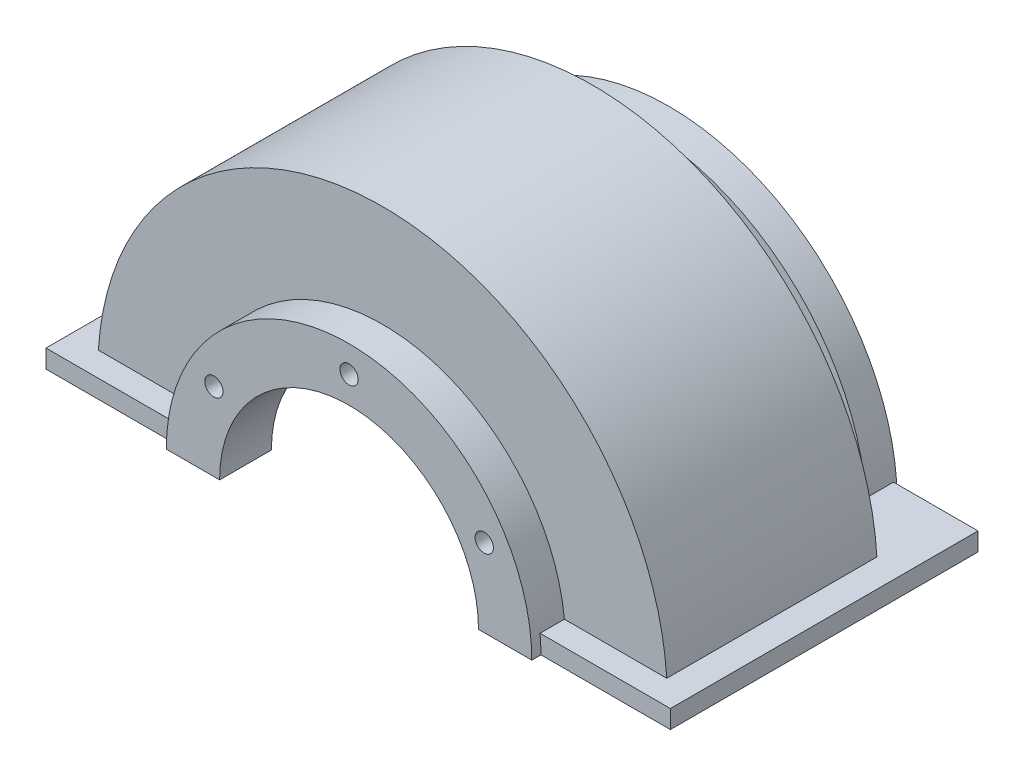
from build123d import *

# Parameters (mm, degrees)
BOSS_EXTRUDE1_DEPTH            = 202
CUT_EXTRUDE1_START             = -16
CUT_EXTRUDE1_DEPTH             = 16
CUT_EXTRUDE2_DEPTH             = 18
CUT_EXTRUDE3_DEPTH             = 30
BOSS_EXTRUDE2_START            = 2
BOSS_EXTRUDE2_DEPTH            = 2
BOSS_EXTRUDE3_DEPTH            = 6
BOSS_EXTRUDE4_DEPTH            = 30
F_16_0_16_DIAMETER_HOLE1_D     = 16
F_16_0_16_DIAMETER_HOLE1_DEPTH = 20
F_12_0_12_DIAMETER_HOLE1_D     = 12
F_12_0_12_DIAMETER_HOLE1_DEPTH = 34


with BuildPart() as part:
    # Sketch1 → Boss-Extrude1 (new body)
    with BuildSketch(Plane(origin=(0, 0, -358.692981355), x_dir=(-1, 0, 0), z_dir=(0, 0, -1))):
        with BuildLine():
            Line((-707.84521865, 246.743963655), (-726.230642584, 246.743963655))
            Line((-726.230642584, 246.743963655), (-726.230642584, 234.743963655))
            Line((-726.230642584, 234.743963655), (-316.230642584, 234.743963655))
            Line((-316.230642584, 234.743963655), (-316.230642584, 246.743963655))
            Line((-316.230642584, 246.743963655), (-334.616066519, 246.743963655))
            ThreePointArc((-334.616066519, 246.743963655), (-521.230642584, 421.743963655), (-707.84521865, 246.743963655))
        make_face()
    extrude(amount=-BOSS_EXTRUDE1_DEPTH)

    # Sketch2 → Cut-Extrude1 (cut)
    with BuildSketch(Plane.XY.offset(-156.692981355).offset(CUT_EXTRUDE1_START)):
        with BuildLine():
            Line((640.629135037, 246.743963655), (707.84521865, 246.743963655))
            ThreePointArc((707.84521865, 246.743963655), (521.230642584, 421.743963655), (334.616066519, 246.743963655))
            Line((334.616066519, 246.743963655), (401.832150132, 246.743963655))
            ThreePointArc((401.832150132, 246.743963655), (521.230642584, 354.743963655), (640.629135037, 246.743963655))
        make_face()
    extrude(amount=CUT_EXTRUDE1_DEPTH, mode=Mode.SUBTRACT)

    # Sketch3 → Cut-Extrude2 (cut)
    with BuildSketch(Plane(origin=(0, 0, -358.692981355), x_dir=(-1, 0, 0), z_dir=(0, 0, -1))):
        with BuildLine():
            Line((-371.711413052, 246.743963655), (-334.616066519, 246.743963655))
            ThreePointArc((-334.616066519, 246.743963655), (-521.230642584, 421.743963654), (-707.84521865, 246.743963655))
            Line((-707.84521865, 246.743963655), (-670.749872117, 246.743963655))
            ThreePointArc((-670.749872117, 246.743963655), (-521.230642584, 384.743963654), (-371.711413052, 246.743963655))
        make_face()
    extrude(amount=-CUT_EXTRUDE2_DEPTH, mode=Mode.SUBTRACT)

    # Sketch4 → Cut-Extrude3 (cut)
    with BuildSketch(Plane(origin=(0, 0, -340.692981355), x_dir=(-1, 0, 0), z_dir=(0, 0, -1))):
        with BuildLine():
            Line((-707.84521865, 246.743963655), (-334.616066519, 246.743963655))
            ThreePointArc((-334.616066519, 246.743963655), (-521.230642584, 421.743963655), (-707.84521865, 246.743963655))
        make_face()
    extrude(amount=-CUT_EXTRUDE3_DEPTH, mode=Mode.SUBTRACT)

    # Sketch5 → Boss-Extrude2 (add)
    with BuildSketch(Plane(origin=(0, 0, -358.692981355), x_dir=(-1, 0, 0), z_dir=(0, 0, -1)).offset(BOSS_EXTRUDE2_START)):
        with BuildLine():
            Line((-371.230642584, 234.743963655), (-671.230642584, 234.743963655))
            ThreePointArc((-671.230642584, 234.743963655), (-521.230642584, 384.743963655), (-371.230642584, 234.743963655))
        make_face()
    extrude(amount=-BOSS_EXTRUDE2_DEPTH)

    # Sketch6 → Boss-Extrude3 (add)
    with BuildSketch(Plane.XY.offset(-156.692981355)):
        with BuildLine():
            Line((641.230642584, 234.743963655), (401.230642584, 234.743963655))
            ThreePointArc((401.230642584, 234.743963655), (521.230642584, 354.743963655), (641.230642584, 234.743963655))
        make_face()
    extrude(amount=BOSS_EXTRUDE3_DEPTH)

    # Sketch7 → Boss-Extrude4 (add)
    with BuildSketch(Plane.XY.offset(-340.692981355)):
        with BuildLine():
            Line((619.500678709, 246.743963655), (422.960606459, 246.743963655))
            ThreePointArc((422.960606459, 246.743963655), (521.230642584, 333.743963655), (619.500678709, 246.743963655))
        make_face()
    extrude(amount=BOSS_EXTRUDE4_DEPTH)

    # Sketch8 → Cut-Revolve1 (revolve, cut)
    with BuildSketch(Plane(origin=(0, 234.743963655, 0), x_dir=(1, 0, 0), z_dir=(0, 1, 0))):
        Polygon((606.230642584, 360.692981355), (521.230642584, 360.692981355), (521.230642584, 150.692981355), (606.230642584, 150.692981355), (606.230642584, 184.692981355), (696.230642584, 184.692981355), (696.230642584, 298.692981355), (606.230642584, 298.692981355), align=None)
    revolve(axis=Axis((521.230642584, 234.743963655, -360.692981355), (0, 0, 1)), mode=Mode.SUBTRACT)

    # Ø16.0 (16) diameter hole1
    with Locations(Plane.XY.offset(-340.692981355)):
        with Locations((421.637721149, 292.243963655), (620.82356402, 292.243963655)):
            Hole(F_16_0_16_DIAMETER_HOLE1_D / 2, depth=F_16_0_16_DIAMETER_HOLE1_DEPTH)

    # Ø12.0 (12) diameter hole1
    with Locations(Plane.XY.offset(-150.692981355)):
        with Locations((521.230642584, 337.243963655), (432.463038696, 285.993963655), (609.998246472, 285.993963655)):
            Hole(F_12_0_12_DIAMETER_HOLE1_D / 2, depth=F_12_0_12_DIAMETER_HOLE1_DEPTH)


solid = part.part
